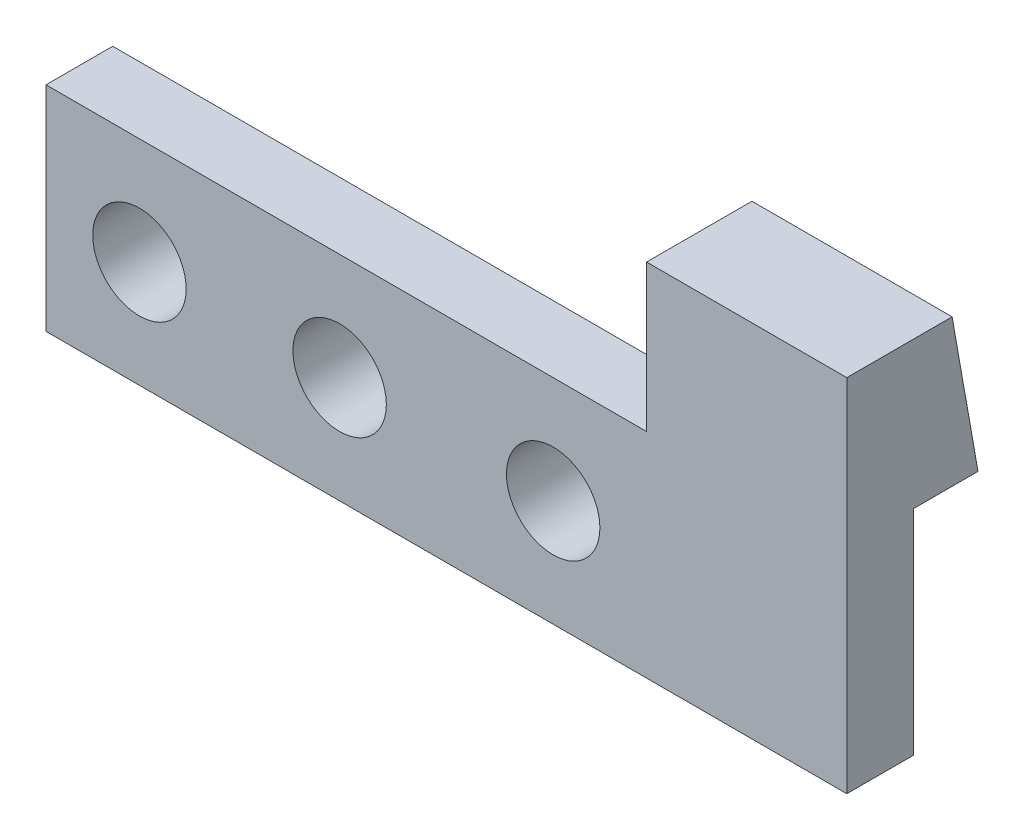
SolidWorks part; units mm, degrees
ref_plane "Front Plane" through (0, 0, 0) normal (0, 0, 1) x (1, 0, 0)
ref_plane "Top Plane" through (0, 0, 0) normal (0, 1, 0) x (1, 0, 0)
ref_plane "Right Plane" through (0, 0, 0) normal (1, 0, 0) x (0, 0, -1)
sketch "Sketch1" plane through (0, 0, 0) normal (1, 0, 0) x (0, 0, -1)
  line L0 (0, 0) -> (0, 27)
  line L1 (0, 27) -> (7.8903, 27)
  line L2 (7.8903, 27) -> (9.8299, 16)
  line L3 (9.8299, 16) -> (5, 16)
  line L4 (5, 16) -> (5, 0)
  line L5 (5, 0) -> (0, 0)
  dimension "D1" = 5
  dimension "D2" = 27
  dimension "D3" = 7.8903
  dimension "D4" = 16
  dimension "D5" = 11.1697
extrude "Boss-Extrude1" add sketch "Sketch1" along normal blind 60
ref_plane "Plane1" through (0, 0, 0) normal (0, 0, 1) x (1, 0, 0)
sketch "Sketch2" plane through (0, 0, 0) normal (0, 0, 1) x (1, 0, 0)
  line L1 (0, 27) -> (45, 27)
  line L2 (0, 27) -> (0, 16)
  line L3 (0, 16) -> (45, 16)
  line L4 (45, 27) -> (45, 16)
  dimension "D1" = 45
  dimension "D2" = 11
extrude "Cut-Extrude1" cut sketch "Sketch2" against normal blind 60
ref_plane "Plane2" through (0, 0, 0) normal (0, 0, 1) x (1, 0, 0)
sketch "Sketch3" plane through (0, 0, 0) normal (0, 0, 1) x (1, 0, 0)
  line L0 (0, 8) -> (60, 8) construction
  line L1 (0, 16) -> (0, 0) construction
  line L2 (60, 27) -> (60, 0) construction
  circle A0 centre (7, 8) radius 3.5
  circle A1 centre (22, 8) radius 3.5
  circle A2 centre (38, 8) radius 3.5
  dimension "D1" = 7
  dimension "D2" = 15
  dimension "D3" = 16
extrude "Cut-Extrude2" cut sketch "Sketch3" against normal blind 60
